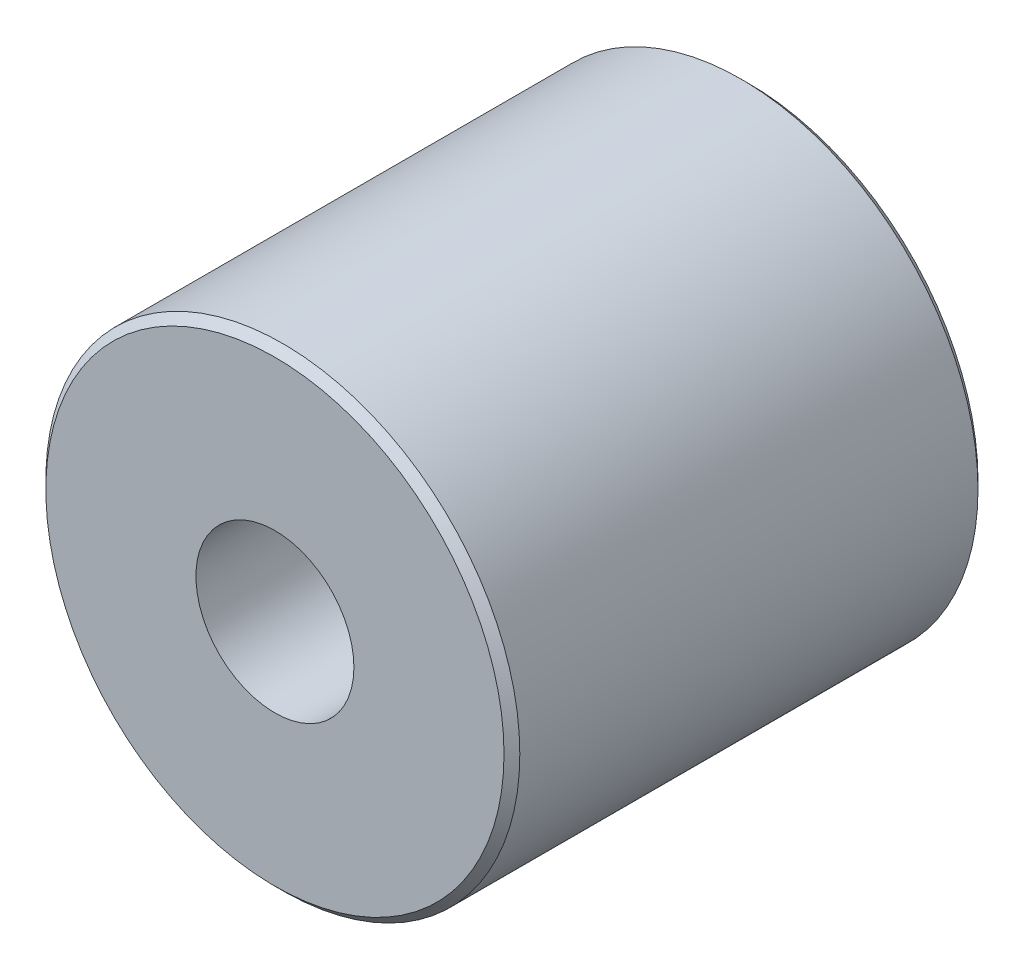
SolidWorks part; units mm, degrees
material "1023 碳钢板 (SS)"
ref_plane "Front Plane" through (0, 0, 0) normal (0, 0, 1) x (1, 0, 0)
ref_plane "Top Plane" through (0, 0, 0) normal (0, 1, 0) x (1, 0, 0)
ref_plane "Right Plane" through (0, 0, 0) normal (1, 0, 0) x (0, 0, -1)
sketch "Sketch1" plane through (0, 0, 0) normal (0, 0, 1) x (1, 0, 0)
  circle A0 centre (0, 0) radius 15
  circle A1 centre (0, 0) radius 5
  dimension "D1" = 30
  dimension "D2" = 10
extrude "Boss-Extrude1" add sketch "Sketch1" along normal blind 30
chamfer "Chamfer1" distance 0.5 angle 45 2 edges at (15, 0, 0) (15, 0, 30)
